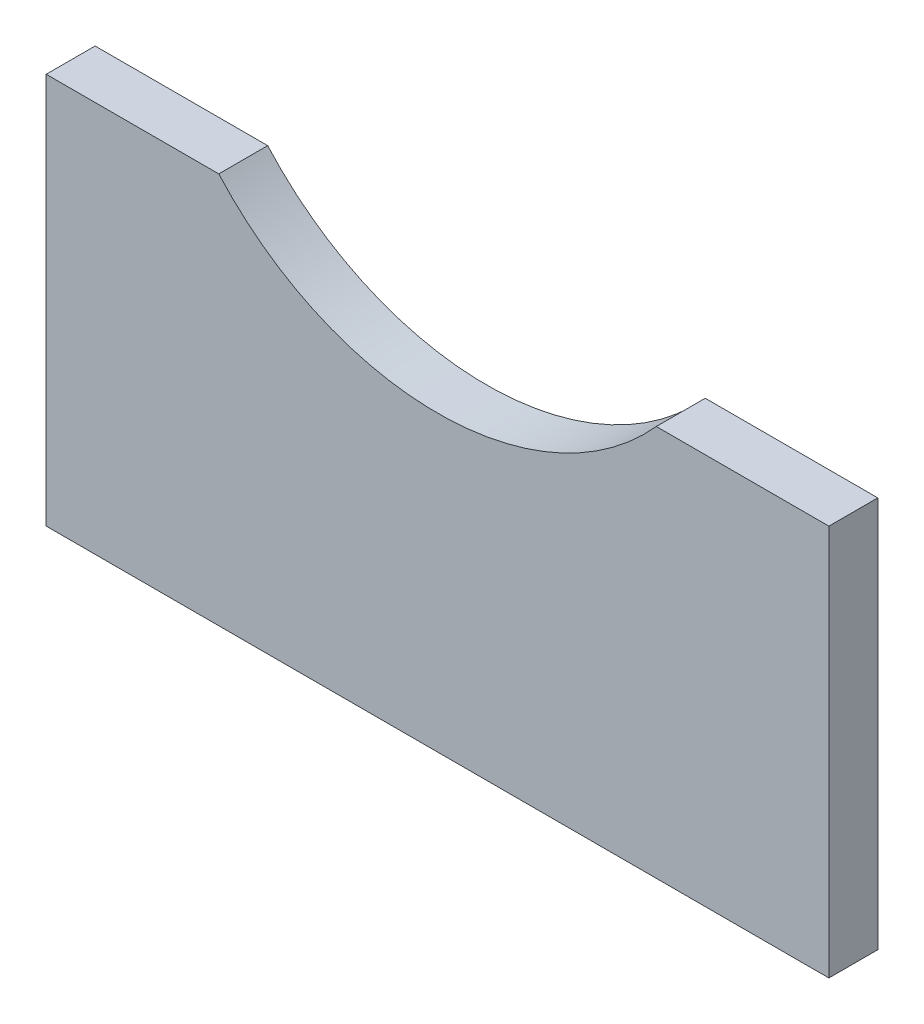
SolidWorks part; units mm, degrees
ref_plane "Front Plane" through (0, 0, 0) normal (0, 0, 1) x (1, 0, 0)
ref_plane "Top Plane" through (0, 0, 0) normal (0, 1, 0) x (1, 0, 0)
ref_plane "Right Plane" through (0, 0, 0) normal (1, 0, 0) x (0, 0, -1)
sketch "Sketch1" plane through (0, 0, 133.35) normal (0, 0, 1) x (1, 0, 0)
  line L0 (0, -38.1) -> (0, -128.9021) construction
  line L1 (-76.2, -38.1) -> (-42.5971, -38.1)
  line L2 (-76.2, -38.1) -> (-76.2, -114.3)
  line L3 (-76.2, -114.3) -> (76.2, -114.3)
  line L4 (76.2, -38.1) -> (76.2, -114.3)
  line L5 (42.5971, -38.1) -> (76.2, -38.1)
  circle A0 centre (0, 0) radius 57.15 construction
  arc A1 (-42.5971, -38.1) -> (42.5971, -38.1) centre (0, 0) ccw
  dimension "D1" = 152.4
extrude "Boss-Extrude1" add sketch "Sketch1" against normal up to vertex (9.525 mm away)
